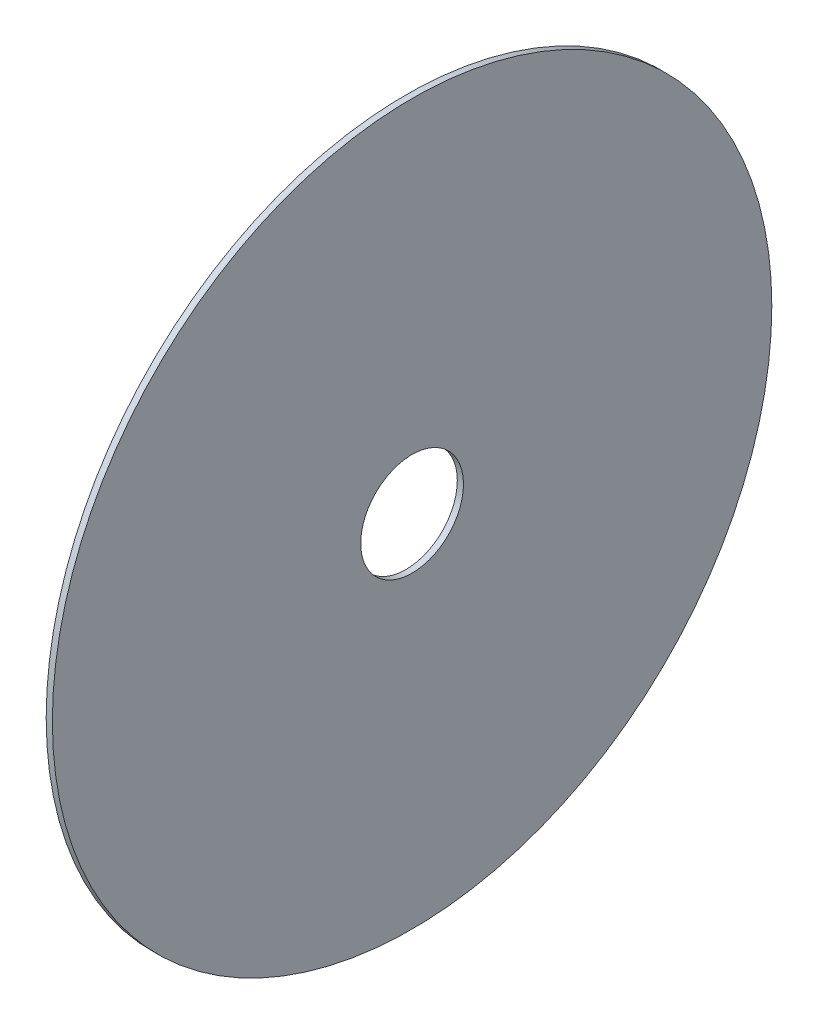
SolidWorks part; units mm, degrees
material "普通碳钢"
ref_plane "Front Plane" through (0, 0, 0) normal (0, 0, 1) x (1, 0, 0)
ref_plane "Top Plane" through (0, 0, 0) normal (0, 1, 0) x (1, 0, 0)
ref_plane "Right Plane" through (0, 0, 0) normal (1, 0, 0) x (0, 0, -1)
ref_plane "Plane1" through (-2, 0, 0) normal (-1, 0, 0) x (0, -1, 0)
sketch "Sketch1" plane through (-2, 0, 0) normal (-1, 0, 0) x (0, -1, 0)
  line L0 (8.1286, -199.8347) -> (3.6487, -192.0754)
  line L1 (5.2808, -190.9326) -> (12.5581, -199.6053)
  line L2 (69.4831, -187.5423) -> (62.8247, -181.547)
  line L3 (64.0237, -179.9558) -> (73.6249, -185.9553)
  line L4 (124.0361, -156.8918) -> (115.8509, -153.2476)
  line L5 (116.4996, -151.3637) -> (127.4848, -154.1026)
  line L6 (166.4476, -110.8837) -> (157.5369, -109.9472)
  line L7 (157.5717, -107.9551) -> (168.8656, -107.1654)
  line L8 (192.566, -54.0216) -> (183.802, -55.8844)
  line L9 (183.2195, -53.9791) -> (193.7166, -49.738)
  line L10 (199.8347, 8.1286) -> (192.0754, 3.6487)
  line L11 (190.9326, 5.2808) -> (199.6053, 12.5581)
  line L12 (187.5423, 69.4831) -> (181.547, 62.8247)
  line L13 (179.9558, 64.0237) -> (185.9553, 73.6249)
  line L14 (156.8918, 124.0361) -> (153.2476, 115.8509)
  line L15 (151.3637, 116.4996) -> (154.1026, 127.4848)
  line L16 (110.8837, 166.4476) -> (109.9472, 157.5369)
  line L17 (107.9551, 157.5717) -> (107.1654, 168.8656)
  line L18 (54.0216, 192.566) -> (55.8844, 183.802)
  line L19 (53.9791, 183.2195) -> (49.738, 193.7166)
  line L20 (-8.1286, 199.8347) -> (-3.6487, 192.0754)
  line L21 (-5.2808, 190.9326) -> (-12.5581, 199.6053)
  line L22 (-69.4831, 187.5423) -> (-62.8247, 181.547)
  line L23 (-64.0237, 179.9558) -> (-73.6249, 185.9553)
  line L24 (-124.0361, 156.8918) -> (-115.8509, 153.2476)
  line L25 (-116.4996, 151.3637) -> (-127.4848, 154.1026)
  line L26 (-166.4476, 110.8837) -> (-157.5369, 109.9472)
  line L27 (-157.5717, 107.9551) -> (-168.8656, 107.1654)
  line L28 (-192.566, 54.0216) -> (-183.802, 55.8844)
  line L29 (-183.2195, 53.9791) -> (-193.7166, 49.738)
  line L30 (-199.8347, -8.1286) -> (-192.0754, -3.6487)
  line L31 (-190.9326, -5.2808) -> (-199.6053, -12.5581)
  line L32 (-187.5423, -69.4831) -> (-181.547, -62.8247)
  line L33 (-179.9558, -64.0237) -> (-185.9553, -73.6249)
  line L34 (-156.8918, -124.0361) -> (-153.2476, -115.8509)
  line L35 (-151.3637, -116.4996) -> (-154.1026, -127.4848)
  line L36 (-110.8837, -166.4476) -> (-109.9472, -157.5369)
  line L37 (-107.9551, -157.5717) -> (-107.1654, -168.8656)
  line L38 (-54.0216, -192.566) -> (-55.8844, -183.802)
  line L39 (-53.9791, -183.2195) -> (-49.738, -193.7166)
  arc A0 (-49.738, -193.7166) -> (8.1286, -199.8347) centre (0, 0) ccw
  arc A1 (3.6487, -192.0754) -> (5.2808, -190.9326) centre (4.5147, -191.5754) cw
  arc A2 (12.5581, -199.6053) -> (69.4831, -187.5423) centre (0, 0) ccw
  arc A3 (62.8247, -181.547) -> (64.0237, -179.9558) centre (63.4938, -180.8039) cw
  arc A4 (73.6249, -185.9553) -> (124.0361, -156.8918) centre (0, 0) ccw
  arc A5 (115.8509, -153.2476) -> (116.4996, -151.3637) centre (116.2577, -152.334) cw
  arc A6 (127.4848, -154.1026) -> (166.4476, -110.8837) centre (0, 0) ccw
  arc A7 (157.5369, -109.9472) -> (157.5717, -107.9551) centre (157.6414, -108.9527) cw
  arc A8 (168.8656, -107.1654) -> (192.566, -54.0216) centre (0, 0) ccw
  arc A9 (183.802, -55.8844) -> (183.2195, -53.9791) centre (183.5941, -54.9063) cw
  arc A10 (193.7166, -49.738) -> (199.8347, 8.1286) centre (0, 0) ccw
  arc A11 (192.0754, 3.6487) -> (190.9326, 5.2808) centre (191.5754, 4.5147) cw
  arc A12 (199.6053, 12.5581) -> (187.5423, 69.4831) centre (0, 0) ccw
  arc A13 (181.547, 62.8247) -> (179.9558, 64.0237) centre (180.8039, 63.4938) cw
  arc A14 (185.9553, 73.6249) -> (156.8918, 124.0361) centre (0, 0) ccw
  arc A15 (153.2476, 115.8509) -> (151.3637, 116.4996) centre (152.334, 116.2577) cw
  arc A16 (154.1026, 127.4848) -> (110.8837, 166.4476) centre (0, 0) ccw
  arc A17 (109.9472, 157.5369) -> (107.9551, 157.5717) centre (108.9527, 157.6414) cw
  arc A18 (107.1654, 168.8656) -> (54.0216, 192.566) centre (0, 0) ccw
  arc A19 (55.8844, 183.802) -> (53.9791, 183.2195) centre (54.9063, 183.5941) cw
  arc A20 (49.738, 193.7166) -> (-8.1286, 199.8347) centre (0, 0) ccw
  arc A21 (-3.6487, 192.0754) -> (-5.2808, 190.9326) centre (-4.5147, 191.5754) cw
  arc A22 (-12.5581, 199.6053) -> (-69.4831, 187.5423) centre (0, 0) ccw
  arc A23 (-62.8247, 181.547) -> (-64.0237, 179.9558) centre (-63.4938, 180.8039) cw
  arc A24 (-73.6249, 185.9553) -> (-124.0361, 156.8918) centre (0, 0) ccw
  arc A25 (-115.8509, 153.2476) -> (-116.4996, 151.3637) centre (-116.2577, 152.334) cw
  arc A26 (-127.4848, 154.1026) -> (-166.4476, 110.8837) centre (0, 0) ccw
  arc A27 (-157.5369, 109.9472) -> (-157.5717, 107.9551) centre (-157.6414, 108.9527) cw
  arc A28 (-168.8656, 107.1654) -> (-192.566, 54.0216) centre (0, 0) ccw
  arc A29 (-183.802, 55.8844) -> (-183.2195, 53.9791) centre (-183.5941, 54.9063) cw
  arc A30 (-193.7166, 49.738) -> (-199.8347, -8.1286) centre (0, 0) ccw
  arc A31 (-192.0754, -3.6487) -> (-190.9326, -5.2808) centre (-191.5754, -4.5147) cw
  arc A32 (-199.6053, -12.5581) -> (-187.5423, -69.4831) centre (0, 0) ccw
  arc A33 (-181.547, -62.8247) -> (-179.9558, -64.0237) centre (-180.8039, -63.4938) cw
  arc A34 (-185.9553, -73.6249) -> (-156.8918, -124.0361) centre (0, 0) ccw
  arc A35 (-153.2476, -115.8509) -> (-151.3637, -116.4996) centre (-152.334, -116.2577) cw
  arc A36 (-154.1026, -127.4848) -> (-110.8837, -166.4476) centre (0, 0) ccw
  arc A37 (-109.9472, -157.5369) -> (-107.9551, -157.5717) centre (-108.9527, -157.6414) cw
  arc A38 (-107.1654, -168.8656) -> (-54.0216, -192.566) centre (0, 0) ccw
  arc A39 (-55.8844, -183.802) -> (-53.9791, -183.2195) centre (-54.9063, -183.5941) cw
extrude "Boss-Extrude1" add sketch "Sketch1" against normal blind 4
sketch "Sketch2" plane through (2, 0, 0) normal (1, 0, 0) x (0, 0, -1)
  line L0 (181.547, -62.8247) -> (181.845, -63.1557)
  line L1 (192.3901, -6.5038) -> (190.9326, -5.2808)
  line L2 (192.0754, -3.6487) -> (192.4611, -3.8714)
  line L3 (184.9836, 53.2663) -> (183.2195, 53.9791)
  line L4 (183.802, 55.8844) -> (184.2377, 55.7918)
  line L5 (159.4697, 107.8224) -> (157.5717, 107.9551)
  line L6 (157.5369, 109.9472) -> (157.9798, 109.9937)
  line L7 (118.3457, 151.824) -> (116.4996, 151.3637)
  line L8 (115.8509, 153.2476) -> (116.2578, 153.4287)
  line L9 (65.6373, 180.9641) -> (64.0237, 179.9558)
  line L10 (62.8247, 181.547) -> (63.1557, 181.845)
  line L11 (6.5038, 192.3901) -> (5.2808, 190.9326)
  line L12 (3.6487, 192.0754) -> (3.8714, 192.4611)
  line L13 (-53.2663, 184.9836) -> (-53.9791, 183.2195)
  line L14 (-55.8844, 183.802) -> (-55.7918, 184.2377)
  line L15 (-107.8224, 159.4697) -> (-107.9551, 157.5717)
  line L16 (-109.9472, 157.5369) -> (-109.9937, 157.9798)
  line L17 (-151.824, 118.3457) -> (-151.3637, 116.4996)
  line L18 (-153.2476, 115.8509) -> (-153.4287, 116.2578)
  line L19 (-180.9641, 65.6373) -> (-179.9558, 64.0237)
  line L20 (-181.547, 62.8247) -> (-181.845, 63.1557)
  line L21 (-192.3901, 6.5038) -> (-190.9326, 5.2808)
  line L22 (-192.0754, 3.6487) -> (-192.4611, 3.8714)
  line L23 (-184.9836, -53.2663) -> (-183.2195, -53.9791)
  line L24 (-183.802, -55.8844) -> (-184.2377, -55.7918)
  line L25 (-159.4697, -107.8224) -> (-157.5717, -107.9551)
  line L26 (-157.5369, -109.9472) -> (-157.9798, -109.9937)
  line L27 (-118.3457, -151.824) -> (-116.4996, -151.3637)
  line L28 (-115.8509, -153.2476) -> (-116.2578, -153.4287)
  line L29 (-65.6373, -180.9641) -> (-64.0237, -179.9558)
  line L30 (-62.8247, -181.547) -> (-63.1557, -181.845)
  line L31 (-6.5038, -192.3901) -> (-5.2808, -190.9326)
  line L32 (-3.6487, -192.0754) -> (-3.8714, -192.4611)
  line L33 (53.2663, -184.9836) -> (53.9791, -183.2195)
  line L34 (55.8844, -183.802) -> (55.7918, -184.2377)
  line L35 (107.8224, -159.4697) -> (107.9551, -157.5717)
  line L36 (109.9472, -157.5369) -> (109.9937, -157.9798)
  line L37 (151.824, -118.3457) -> (151.3637, -116.4996)
  line L38 (153.2476, -115.8509) -> (153.4287, -116.2578)
  line L39 (180.9641, -65.6373) -> (179.9558, -64.0237)
  arc A0 (179.9558, -64.0237) -> (181.547, -62.8247) centre (180.8039, -63.4938) cw
  arc A1 (181.845, -63.1557) -> (192.3901, -6.5038) centre (0, 0) ccw
  arc A2 (190.9326, -5.2808) -> (192.0754, -3.6487) centre (191.5754, -4.5147) cw
  arc A3 (192.4611, -3.8714) -> (184.9836, 53.2663) centre (0, 0) ccw
  arc A4 (183.2195, 53.9791) -> (183.802, 55.8844) centre (183.5941, 54.9063) cw
  arc A5 (184.2377, 55.7918) -> (159.4697, 107.8224) centre (0, 0) ccw
  arc A6 (157.5717, 107.9551) -> (157.5369, 109.9472) centre (157.6414, 108.9527) cw
  arc A7 (157.9798, 109.9937) -> (118.3457, 151.824) centre (0, 0) ccw
  arc A8 (116.4996, 151.3637) -> (115.8509, 153.2476) centre (116.2577, 152.334) cw
  arc A9 (116.2578, 153.4287) -> (65.6373, 180.9641) centre (0, 0) ccw
  arc A10 (64.0237, 179.9558) -> (62.8247, 181.547) centre (63.4938, 180.8039) cw
  arc A11 (63.1557, 181.845) -> (6.5038, 192.3901) centre (0, 0) ccw
  arc A12 (5.2808, 190.9326) -> (3.6487, 192.0754) centre (4.5147, 191.5754) cw
  arc A13 (3.8714, 192.4611) -> (-53.2663, 184.9836) centre (0, 0) ccw
  arc A14 (-53.9791, 183.2195) -> (-55.8844, 183.802) centre (-54.9063, 183.5941) cw
  arc A15 (-55.7918, 184.2377) -> (-107.8224, 159.4697) centre (0, 0) ccw
  arc A16 (-107.9551, 157.5717) -> (-109.9472, 157.5369) centre (-108.9527, 157.6414) cw
  arc A17 (-109.9937, 157.9798) -> (-151.824, 118.3457) centre (0, 0) ccw
  arc A18 (-151.3637, 116.4996) -> (-153.2476, 115.8509) centre (-152.334, 116.2577) cw
  arc A19 (-153.4287, 116.2578) -> (-180.9641, 65.6373) centre (0, 0) ccw
  arc A20 (-179.9558, 64.0237) -> (-181.547, 62.8247) centre (-180.8039, 63.4938) cw
  arc A21 (-181.845, 63.1557) -> (-192.3901, 6.5038) centre (0, 0) ccw
  arc A22 (-190.9326, 5.2808) -> (-192.0754, 3.6487) centre (-191.5754, 4.5147) cw
  arc A23 (-192.4611, 3.8714) -> (-184.9836, -53.2663) centre (0, 0) ccw
  arc A24 (-183.2195, -53.9791) -> (-183.802, -55.8844) centre (-183.5941, -54.9063) cw
  arc A25 (-184.2377, -55.7918) -> (-159.4697, -107.8224) centre (0, 0) ccw
  arc A26 (-157.5717, -107.9551) -> (-157.5369, -109.9472) centre (-157.6414, -108.9527) cw
  arc A27 (-157.9798, -109.9937) -> (-118.3457, -151.824) centre (0, 0) ccw
  arc A28 (-116.4996, -151.3637) -> (-115.8509, -153.2476) centre (-116.2577, -152.334) cw
  arc A29 (-116.2578, -153.4287) -> (-65.6373, -180.9641) centre (0, 0) ccw
  arc A30 (-64.0237, -179.9558) -> (-62.8247, -181.547) centre (-63.4938, -180.8039) cw
  arc A31 (-63.1557, -181.845) -> (-6.5038, -192.3901) centre (0, 0) ccw
  arc A32 (-5.2808, -190.9326) -> (-3.6487, -192.0754) centre (-4.5147, -191.5754) cw
  arc A33 (-3.8714, -192.4611) -> (53.2663, -184.9836) centre (0, 0) ccw
  arc A34 (53.9791, -183.2195) -> (55.8844, -183.802) centre (54.9063, -183.5941) cw
  arc A35 (55.7918, -184.2377) -> (107.8224, -159.4697) centre (0, 0) ccw
  arc A36 (107.9551, -157.5717) -> (109.9472, -157.5369) centre (108.9527, -157.6414) cw
  arc A37 (109.9937, -157.9798) -> (151.824, -118.3457) centre (0, 0) ccw
  arc A38 (151.3637, -116.4996) -> (153.2476, -115.8509) centre (152.334, -116.2577) cw
  arc A39 (153.4287, -116.2578) -> (180.9641, -65.6373) centre (0, 0) ccw
extrude "Cut-Extrude1" cut sketch "Sketch2" against normal blind 0.7
sketch "Sketch3" plane through (-2, 0, 0) normal (-1, 0, 0) x (0, 0, 1)
  line L0 (-190.9326, -5.2808) -> (-199.6053, -12.5581)
  line L1 (-187.5423, -69.4831) -> (-181.547, -62.8247)
  line L2 (-179.9558, -64.0237) -> (-180.9641, -65.6373)
  line L3 (-153.4287, -116.2578) -> (-153.2476, -115.8509)
  line L4 (-151.3637, -116.4996) -> (-151.824, -118.3457)
  line L5 (-109.9937, -157.9798) -> (-109.9472, -157.5369)
  line L6 (-107.9551, -157.5717) -> (-107.8224, -159.4697)
  line L7 (-55.7918, -184.2377) -> (-55.8844, -183.802)
  line L8 (-53.9791, -183.2195) -> (-53.2663, -184.9836)
  line L9 (3.8714, -192.4611) -> (3.6487, -192.0754)
  line L10 (5.2808, -190.9326) -> (6.5038, -192.3901)
  line L11 (63.1557, -181.845) -> (62.8247, -181.547)
  line L12 (64.0237, -179.9558) -> (65.6373, -180.9641)
  line L13 (116.2578, -153.4287) -> (115.8509, -153.2476)
  line L14 (116.4996, -151.3637) -> (118.3457, -151.824)
  line L15 (157.9798, -109.9937) -> (157.5369, -109.9472)
  line L16 (157.5717, -107.9551) -> (159.4697, -107.8224)
  line L17 (184.2377, -55.7918) -> (183.802, -55.8844)
  line L18 (183.2195, -53.9791) -> (184.9836, -53.2663)
  line L19 (192.4611, 3.8714) -> (192.0754, 3.6487)
  line L20 (190.9326, 5.2808) -> (192.3901, 6.5038)
  line L21 (181.845, 63.1557) -> (181.547, 62.8247)
  line L22 (179.9558, 64.0237) -> (180.9641, 65.6373)
  line L23 (153.4287, 116.2578) -> (153.2476, 115.8509)
  line L24 (151.3637, 116.4996) -> (151.824, 118.3457)
  line L25 (109.9937, 157.9798) -> (109.9472, 157.5369)
  line L26 (107.9551, 157.5717) -> (107.8224, 159.4697)
  line L27 (55.7918, 184.2377) -> (55.8844, 183.802)
  line L28 (53.9791, 183.2195) -> (53.2663, 184.9836)
  line L29 (-3.8714, 192.4611) -> (-3.6487, 192.0754)
  line L30 (-5.2808, 190.9326) -> (-6.5038, 192.3901)
  line L31 (-63.1557, 181.845) -> (-62.8247, 181.547)
  line L32 (-64.0237, 179.9558) -> (-65.6373, 180.9641)
  line L33 (-116.2578, 153.4287) -> (-115.8509, 153.2476)
  line L34 (-116.4996, 151.3637) -> (-118.3457, 151.824)
  line L35 (-157.9798, 109.9937) -> (-157.5369, 109.9472)
  line L36 (-157.5717, 107.9551) -> (-159.4697, 107.8224)
  line L37 (-184.2377, 55.7918) -> (-183.802, 55.8844)
  line L38 (-183.2195, 53.9791) -> (-184.9836, 53.2663)
  line L39 (-192.4611, -3.8714) -> (-192.0754, -3.6487)
  arc A0 (-199.6053, -12.5581) -> (-187.5423, -69.4831) centre (0, 0) ccw
  arc A1 (-181.547, -62.8247) -> (-179.9558, -64.0237) centre (-180.8039, -63.4938) cw
  arc A2 (-180.9641, -65.6373) -> (-153.4287, -116.2578) centre (0, 0) ccw
  arc A3 (-153.2476, -115.8509) -> (-151.3637, -116.4996) centre (-152.334, -116.2577) cw
  arc A4 (-151.824, -118.3457) -> (-109.9937, -157.9798) centre (0, 0) ccw
  arc A5 (-109.9472, -157.5369) -> (-107.9551, -157.5717) centre (-108.9527, -157.6414) cw
  arc A6 (-107.8224, -159.4697) -> (-55.7918, -184.2377) centre (0, 0) ccw
  arc A7 (-55.8844, -183.802) -> (-53.9791, -183.2195) centre (-54.9063, -183.5941) cw
  arc A8 (-53.2663, -184.9836) -> (3.8714, -192.4611) centre (0, 0) ccw
  arc A9 (3.6487, -192.0754) -> (5.2808, -190.9326) centre (4.5147, -191.5754) cw
  arc A10 (6.5038, -192.3901) -> (63.1557, -181.845) centre (0, 0) ccw
  arc A11 (62.8247, -181.547) -> (64.0237, -179.9558) centre (63.4938, -180.8039) cw
  arc A12 (65.6373, -180.9641) -> (116.2578, -153.4287) centre (0, 0) ccw
  arc A13 (115.8509, -153.2476) -> (116.4996, -151.3637) centre (116.2577, -152.334) cw
  arc A14 (118.3457, -151.824) -> (157.9798, -109.9937) centre (0, 0) ccw
  arc A15 (157.5369, -109.9472) -> (157.5717, -107.9551) centre (157.6414, -108.9527) cw
  arc A16 (159.4697, -107.8224) -> (184.2377, -55.7918) centre (0, 0) ccw
  arc A17 (183.802, -55.8844) -> (183.2195, -53.9791) centre (183.5941, -54.9063) cw
  arc A18 (184.9836, -53.2663) -> (192.4611, 3.8714) centre (0, 0) ccw
  arc A19 (192.0754, 3.6487) -> (190.9326, 5.2808) centre (191.5754, 4.5147) cw
  arc A20 (192.3901, 6.5038) -> (181.845, 63.1557) centre (0, 0) ccw
  arc A21 (181.547, 62.8247) -> (179.9558, 64.0237) centre (180.8039, 63.4938) cw
  arc A22 (180.9641, 65.6373) -> (153.4287, 116.2578) centre (0, 0) ccw
  arc A23 (153.2476, 115.8509) -> (151.3637, 116.4996) centre (152.334, 116.2577) cw
  arc A24 (151.824, 118.3457) -> (109.9937, 157.9798) centre (0, 0) ccw
  arc A25 (109.9472, 157.5369) -> (107.9551, 157.5717) centre (108.9527, 157.6414) cw
  arc A26 (107.8224, 159.4697) -> (55.7918, 184.2377) centre (0, 0) ccw
  arc A27 (55.8844, 183.802) -> (53.9791, 183.2195) centre (54.9063, 183.5941) cw
  arc A28 (53.2663, 184.9836) -> (-3.8714, 192.4611) centre (0, 0) ccw
  arc A29 (-3.6487, 192.0754) -> (-5.2808, 190.9326) centre (-4.5147, 191.5754) cw
  arc A30 (-6.5038, 192.3901) -> (-63.1557, 181.845) centre (0, 0) ccw
  arc A31 (-62.8247, 181.547) -> (-64.0237, 179.9558) centre (-63.4938, 180.8039) cw
  arc A32 (-65.6373, 180.9641) -> (-116.2578, 153.4287) centre (0, 0) ccw
  arc A33 (-115.8509, 153.2476) -> (-116.4996, 151.3637) centre (-116.2577, 152.334) cw
  arc A34 (-118.3457, 151.824) -> (-157.9798, 109.9937) centre (0, 0) ccw
  arc A35 (-157.5369, 109.9472) -> (-157.5717, 107.9551) centre (-157.6414, 108.9527) cw
  arc A36 (-159.4697, 107.8224) -> (-184.2377, 55.7918) centre (0, 0) ccw
  arc A37 (-183.802, 55.8844) -> (-183.2195, 53.9791) centre (-183.5941, 54.9063) cw
  arc A38 (-184.9836, 53.2663) -> (-192.4611, -3.8714) centre (0, 0) ccw
  arc A39 (-192.0754, -3.6487) -> (-190.9326, -5.2808) centre (-191.5754, -4.5147) cw
extrude "Cut-Extrude2" cut sketch "Sketch3" against normal blind 0.3
sketch "Sketch4" plane through (-1.7, 0, 0) normal (-1, 0, 0) x (0, 0, 1)
  line L0 (-199.6053, -12.5581) -> (-192.3901, -6.5038)
  line L1 (-181.845, -63.1557) -> (-187.5423, -69.4831)
  arc A0 (-192.3901, -6.5038) -> (-181.845, -63.1557) centre (0, 0) ccw
  arc A1 (-187.5423, -69.4831) -> (-199.6053, -12.5581) centre (0, 0) cw
extrude "Boss-Extrude2" add sketch "Sketch4" along normal blind 0.3
sketch "Sketch5" plane through (0, 0, 0) normal (0, 0, 1) x (1, 0, 0)
  line L0 (-1.7, 25) -> (-1.7, 0)
  line L1 (-1.7, 0) -> (1.3, 0)
  line L2 (1.3, 0) -> (1.3, 25)
  line L3 (1.3, 25) -> (-1.7, 25)
  line L4 (-1.7, 0) -> (1.3, 0) construction
revolve "Cut-Revolve1" cut sketch "Sketch5" angle 360 about L4
chamfer "Chamfer1" distance 1.13 angle 30 20 edges at (0, 156.8918, -124.0361) (0, 166.4476, 110.8837) (0, -69.4831, -187.5423) (0, -166.4476, -110.8837) (0, 199.8347, -8.1286) (0, -192.566, -54.0216) (0, 54.0216, -192.566) (0, -199.8347, 8.1286) (0, 124.0361, 156.8918) (0, -187.5423, 69.4831) (0, 192.566, 54.0216) (0, -156.8918, 124.0361) (0, 187.5423, -69.4831) (0, -110.8837, 166.4476) (0, 110.8837, -166.4476) (0, -54.0216, 192.566) (0, -8.1286, -199.8347) (0, 8.1286, 199.8347) (0, -124.0361, -156.8918) (0, 69.4831, 187.5423)
sketch "Sketch6" plane through (-2, 0, 0) normal (-1, 0, 0) x (0, 0, 1)
  circle A0 centre (0, 0) radius 175
  dimension "D1" = 350
extrude "Cut-Extrude3" cut sketch "Sketch6" against normal blind 10 flip side to cut
